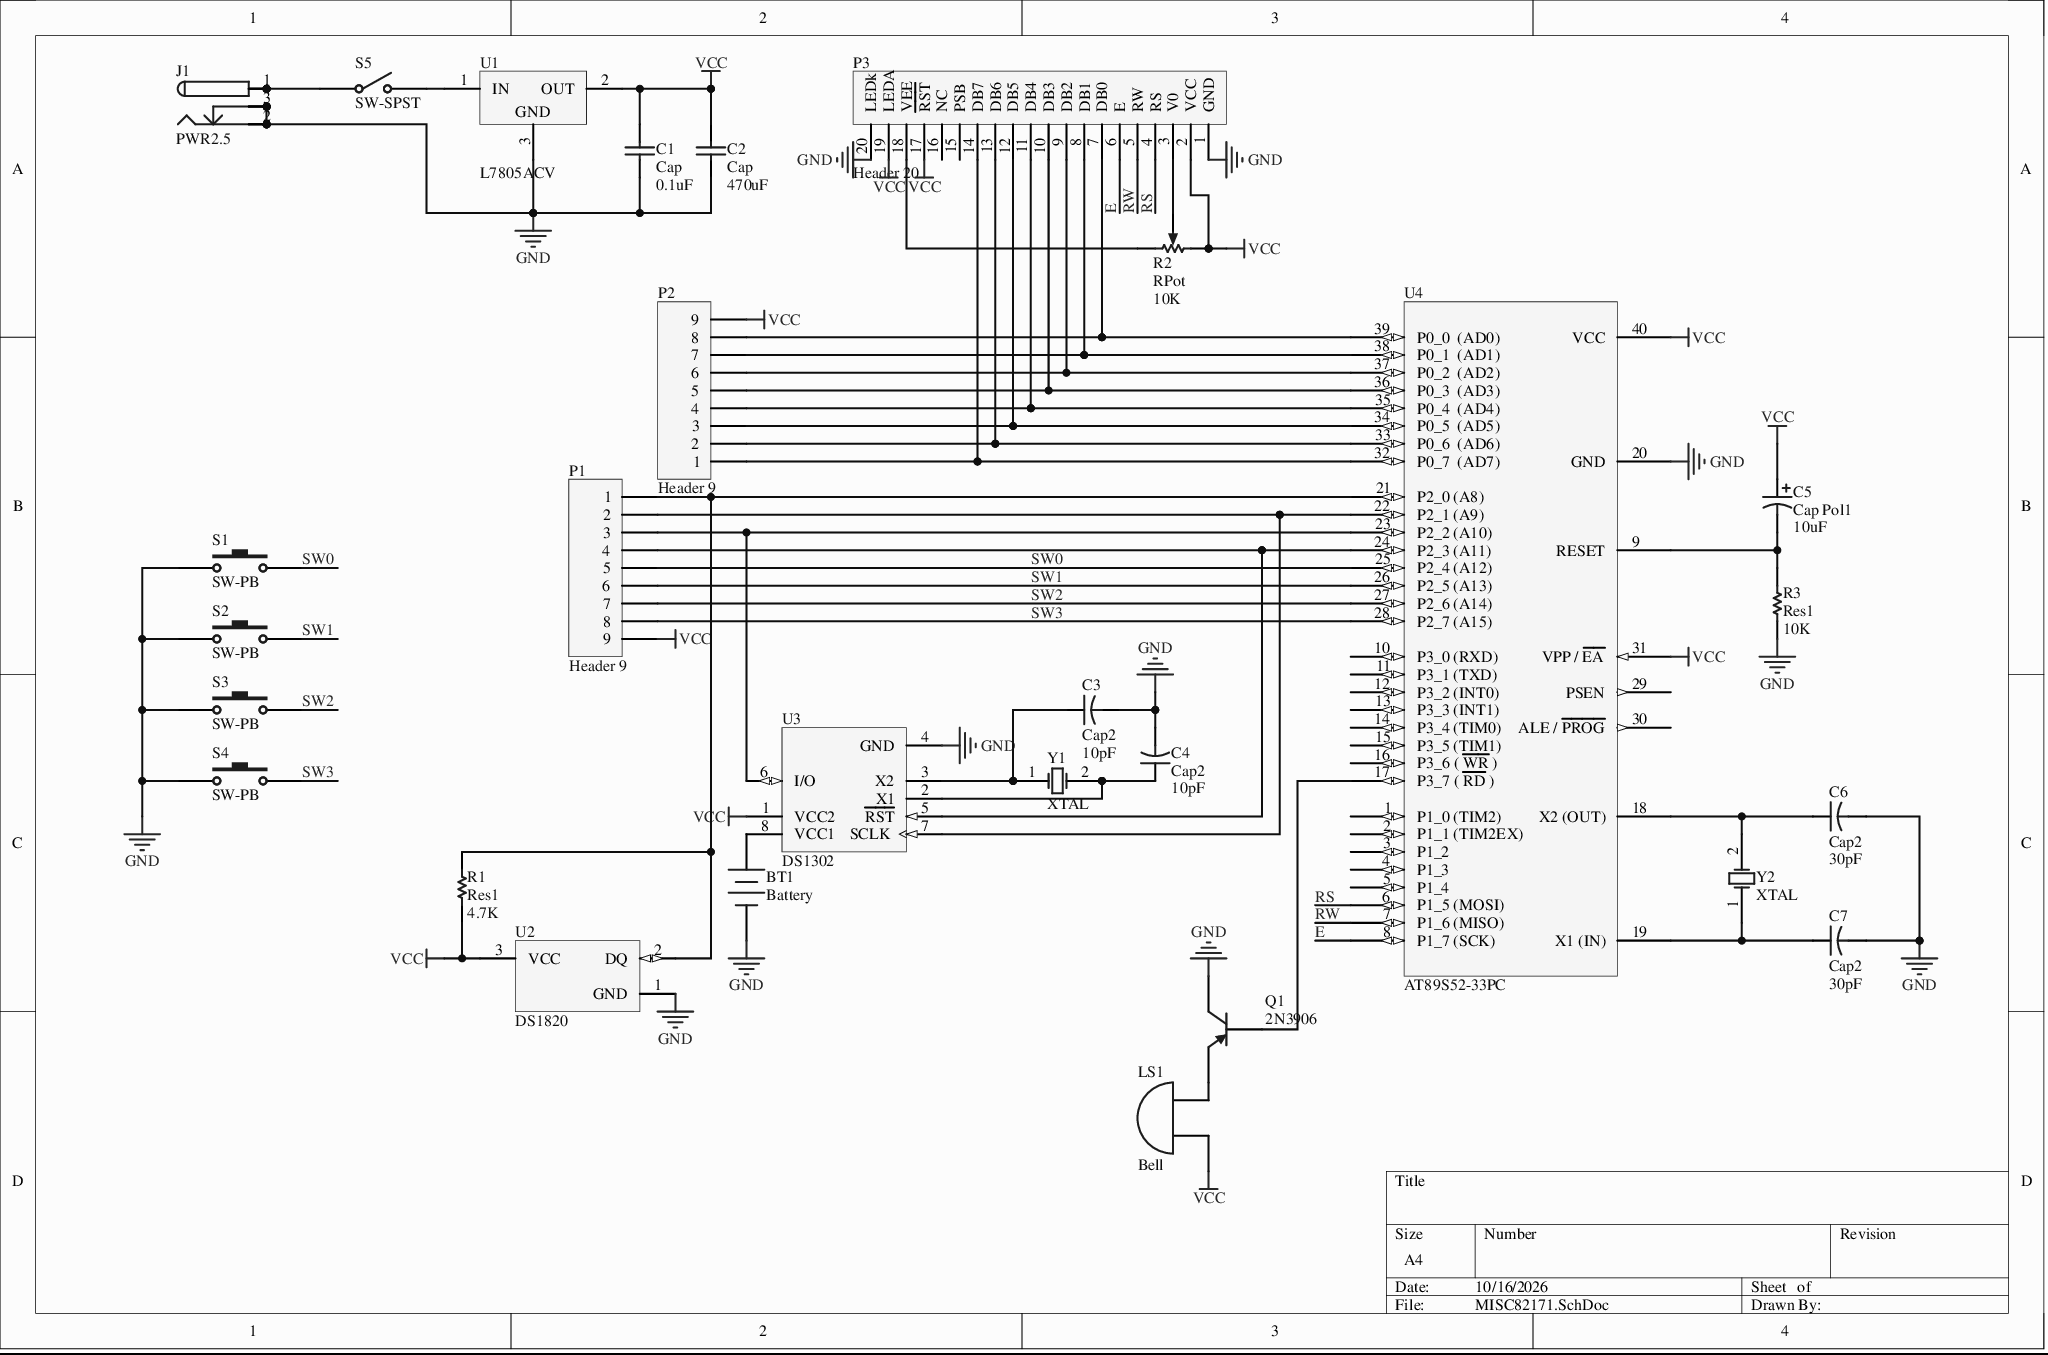
[diagram p0: MISC82171.SchDoc]
# Altium project MISC82171.PrjPcb
1 sheet, 28 parts. Net scope: global (net labels, ports and power ports of the same name join across sheets).
Board file: MISC82171.PcbDoc

## Sheet MISC82171.SchDoc
size A4

### Parts
BT1  Battery  [3V电池]
C1  Cap  value 0.1uF  [RAD-0.3]
C2  Cap  value 470uF  [RAD-0.3]
C3  Cap2  value 10pF  [CAPR5-4X5]
C4  Cap2  value 10pF  [CAPR5-4X5]
C5  Cap Pol1  value 10uF  [RB7.6-15]
C6  Cap2  value 30pF  [CAPR5-4X5]
C7  Cap2  value 30pF  [CAPR5-4X5]
J1  PWR2.5  [DC]
LS1  Bell  [BELL]
P1  Header 9  [HDR1X9]
P2  Header 9  [HDR1X9]
P3  Header 20  [HDR1X20]
Q1  2N3906  [TO-92A]
R1  Res1  value 4.7K  [AXIAL-0.3]
R2  RPot  value 10K  [VR4]
R3  Res1  value 10K  [AXIAL-0.3]
S1  SW-PB  [SW4]
S2  SW-PB  [SW4]
S3  SW-PB  [SW4]
S4  SW-PB  [SW4]
S5  SW-SPST  [SPST-2]
U1  L7805ACV  [TO220ABN]
U2  DS1820  [PR35]
U3  DS1302  [DIP8]
U4  AT89S52-33PC  [DIP40]
Y1  XTAL  [R38]
Y2  XTAL  [XTAL2]

### Nets
GND: BT1.2(-) C1.1 C2.1 C3.2 C4.2 C6.2 C7.2 J1.2 J1.2A J1.2B J1.3 J1.3A J1.3B P3.1(GND) P3.20(LEDk) Q1.3(C) R3.1 S1.1 S2.1 S3.1 S4.1 U1.3(GND) U2.1(GND) U3.4(GND) U4.20(GND)
VCC: C1.2 C2.2 C5.1 LS1.1(A) P1.9 P2.9 P3.2(VCC) P3.17(~{RST}) P3.19(LEDA) R1.1 R2.1(TOP) U1.2(OUT) U2.3(VCC) U3.1(VCC2) U4.31(VPP_/~{_EA}) U4.40(VCC)
E: P3.6(E) U4.8(P1_7_(SCK))
RS: P3.4(RS) U4.6(P1_5_(MOSI))
RW: P3.5(RW) U4.7(P1_6_(MISO))
SW0: P1.5 S1.2 U4.25(P2_4_(A12))
SW1: P1.6 S2.2 U4.26(P2_5_(A13))
SW2: P1.7 S3.2 U4.27(P2_6_(A14))
SW3: P1.8 S4.2 U4.28(P2_7_(A15))
NetBT1_1: BT1.1(+) U3.8(VCC1)
NetC3_1: C3.1 U3.3(X2) Y1.1(OSC1)
NetC4_1: C4.1 U3.2(X1) Y1.2(OSC2)
NetC5_2: C5.2 R3.2 U4.9(RESET)
NetC6_1: C6.1 U4.18(X2_(OUT)) Y2.2(OSC2)
NetC7_1: C7.1 U4.19(X1_(IN)) Y2.1(OSC1)
NetJ1_1: J1.1 J1.1A J1.1B S5.1(COMMON)
NetLS1_2: LS1.2(B) Q1.1(E)
NetP1_1: P1.1 R1.2 U2.2(DQ) U4.21(P2_0_(A8))
NetP1_2: P1.2 U3.7(SCLK) U4.22(P2_1_(A9))
NetP1_3: P1.3 U3.6(I/O) U4.23(P2_2_(A10))
NetP1_4: P1.4 U3.5(~{RST}) U4.24(P2_3_(A11))
NetP2_1: P2.1 P3.14(DB7) U4.32(P0_7__(AD7))
NetP2_2: P2.2 P3.13(DB6) U4.33(P0_6__(AD6))
NetP2_3: P2.3 P3.12(DB5) U4.34(P0_5__(AD5))
NetP2_4: P2.4 P3.11(DB4) U4.35(P0_4__(AD4))
NetP2_5: P2.5 P3.10(DB3) U4.36(P0_3__(AD3))
NetP2_6: P2.6 P3.9(DB2) U4.37(P0_2__(AD2))
NetP2_7: P2.7 P3.8(DB1) U4.38(P0_1__(AD1))
NetP2_8: P2.8 P3.7(DB0) U4.39(P0_0__(AD0))
NetP3_3: P3.3(V0) R2.3(TAP)
NetP3_18: P3.18(VEE) R2.2(BOT)
NetQ1_2: Q1.2(B) U4.17(P3_7_(~{_RD}_))
NetS5_2: S5.2(NO) U1.1(IN)

Not connected (* = marked no-connect by the designer): P3 15(PSB) 16(NC); U4 1(P1_0_(TIM2)) 2(P1_1_(TIM2EX)) 3(P1_2) 4(P1_3) 5(P1_4) 10(P3_0_(RXD)) 11(P3_1_(TXD)) 12(P3_2_(INT0)) 13(P3_3_(INT1)) 14(P3_4_(TIM0)) 15(P3_5_(TIM1)) 16(P3_6_(~{_WR}_)) 29(~{PSEN}) 30(ALE_/~{_PROG})

### Library data of the parts
BT1 = Battery: Multicell Battery; Published: 24-Mar-1999; LatestRevisionDate: 17-Jul-2002; LatestRevisionNote: Re-released for DXP Platform.; PackageReference: BAT-2; PackageDescription: Battery; 2 Leads; Publisher: Altium Limited
C1 C2 = Cap: Capacitor; Published: 8-Jun-2000; LatestRevisionDate: 17-Jul-2002; LatestRevisionNote: Re-released for DXP Platform.; PackageReference: RAD-0.3; PackageDescription: Radial Cap, Thru-Hole; 2 Leads; 0.3 in Pin Spacing; Publisher: Altium Limited
C3 C4 C6 C7 = Cap2: Capacitor; Published: 23-Sep-2002; PackageReference: CAPR5-4X5; PackageDescription: Capacitor; 2 Leads; Publisher: Altium Limited
C5 = Cap Pol1: Polarized Capacitor (Radial); Published: 8-Jun-2000; LatestRevisionDate: 17-Jul-2002; LatestRevisionNote: Re-released for DXP Platform.; PackageReference: RB7.6-15; PackageDescription: Polarized Capacitor (Radial); 2 Leads; Publisher: Altium Limited
J1 = PWR2.5: Low Voltage Power Supply Connector; Published: 17-Dec-2003; DatasheetDocument: 09-May-2002; ComponentLink1Description: Manufacturer Link; Publisher: Altium Limited
LS1 = Bell: Electrical Bell; Published: 24-Mar-1999; LatestRevisionDate: 17-Jul-2002; LatestRevisionNote: Re-released for DXP Platform.; PackageReference: PIN2; Publisher: Altium Limited
P1 P2 = Header 9: Header, 9-Pin; LatestRevisionDate: 17-Jul-2002; LatestRevisionNote: Re-released for DXP Platform.; Publisher: Altium Limited
P3 = Header 20: Header, 20-Pin; LatestRevisionDate: 17-Jul-2002; LatestRevisionNote: Re-released for DXP Platform.; Publisher: Altium Limited
Q1 = 2N3906: PNP General Purpose Amplifier; Published: 8-Jun-2000; LatestRevisionDate: 15-Jan-2003; LatestRevisionNote: PCB Footprint 'BCY-W3/D4.7' replaced; DatasheetVersion: 1997; PackageVersion: Sep-1998; PackageReference: TO-92A; PackageDescription: TO, Flat Index; 3 In-Line, Axial Leads; Body Dia. 4.5mm; Leads 0.51 x 0.48 mm (max); ComponentLink1Description: Manufacturer Link; ComponentLink2Description: Datasheet; ComponentLink2URL: http://www.fairchildsemi.com/ds/2N%2F2N3906.pdf; Publisher: Altium Limited
R1 R3 = Res1: Resistor; Published: 8-Jun-2000; LatestRevisionDate: 17-Jul-2002; LatestRevisionNote: Re-released for DXP Platform.; PackageReference: AXIAL-0.3; PackageDescription: Axial Device, Thru-Hole; 2 Leads; 0.3 in Pin Spacing; Publisher: Altium Limited
R2 = RPot: Potentiometer; Sim Note: Enter the Resistance value and the set point into parameter fields.; Set Position: 0.5; Published: 8-Jun-2000; LatestRevisionDate: 17-Jul-2002; LatestRevisionNote: Re-released for DXP Platform.; PackageReference: VR5; PackageDescription: Variable Resistor, Thru-Hole; 3 Leads; Publisher: Altium Limited
S1-S4 = SW-PB: Switch; Published: 24-Mar-1999; LatestRevisionDate: 17-Jul-2002; LatestRevisionNote: Re-released for DXP Platform.; PackageReference: SPST-2; PackageDescription: Switch; 2 Leads; Publisher: Altium Limited
S5 = SW-SPST: Single-Pole, Single-Throw Switch; Published: 24-Mar-1999; LatestRevisionDate: 17-Jul-2002; LatestRevisionNote: Re-released for DXP Platform.; PackageReference: SPST-2; PackageDescription: Switch; 2 Leads; Publisher: Altium Limited
U1 = L7805ACV: Precision 1A Regulator; Note: Tab is connected to pin 3 (GND).; Published: 24-Aug-2001; LatestRevisionDate: 17-Jul-2002; LatestRevisionNote: Re-released for DXP Platform.; DatasheetVersion: Nov-1999; PackageVersion: Jun-1998; PackageReference: TO220ABN; PackageDescription: TO, Thru-Hole, Vertical, Heatsink Mounted; 3 In-Line Leads; Pitch 2.54 mm; Pin sequence 1, 3, 2; ComponentLink1Description: Manufacturer Link; ComponentLink2Description: Datasheet; ComponentLink2URL: http://www.st.com/stonline/products/literature/ds/2144/l7805ab.pdf; Publisher: Altium Limited
U2 = DS1820: 1-Wire Digital Thermometer; ComponentAvailability: Obsolete; Published: 13-Oct-2000; LatestRevisionDate: 17-Jul-2002; LatestRevisionNote: Re-released for DXP Platform.; DatasheetVersion: 5-Mar-1998; PackageVersion: 1999; PackageReference: PR35; PackageDescription: TO, Flat Index; 3 In-Line, Axial Leads; Body Dia. 4.6mm; Leads 0.56 x 0.51 mm (max); ComponentLink1Description: Manufacturer Link; ComponentLink2Description: Datasheet; ComponentLink2URL: http://pdfserv.maxim-ic.com/en/ds/DS1820-DS1820S.pdf; ComponentLink3Description: Discontinuation Notice; Publisher: Altium Limited
U3 = DS1302: Trickle Charge Timekeeping Chip; Published: 13-Oct-2000; LatestRevisionDate: 17-Jul-2002; LatestRevisionNote: Re-released for DXP Platform.; DatasheetVersion: 2-Jul-1999; PackageVersion: 1999; PackageReference: DIP8; PackageDescription: DIP, 8-Pin, Row Spacing 7.62 mm, Pitch 2.54 mm; ComponentLink1Description: Manufacturer Link; ComponentLink2Description: Datasheet; ComponentLink2URL: http://pdfserv.maxim-ic.com/en/ds/DS1302.pdf; Publisher: Altium Limited
U4 = AT89S52-33PC: Atmel 8 Bit Micro 4.0-5.5V 33MHz 0-70 Deg C 40 PDIP (40P6) Package; GREEN OPTION: NO; Vendor: ATMEL; PartNr: AT89S52-33PC; PackAge: 40P6 40-pin, 0.600" Wide, Plastic Dual Inline Package (PDIP)
Y1 Y2 = XTAL: Crystal Oscillator; Published: 8-Jun-2000; LatestRevisionDate: 17-Jul-2002; LatestRevisionNote: Re-released for DXP Platform.; PackageReference: R38; PackageDescription: Crystal, Thru-Hole; 2 Leads; Body 3.1 x 8.2 mm (Dia.xH); Publisher: Altium Limited